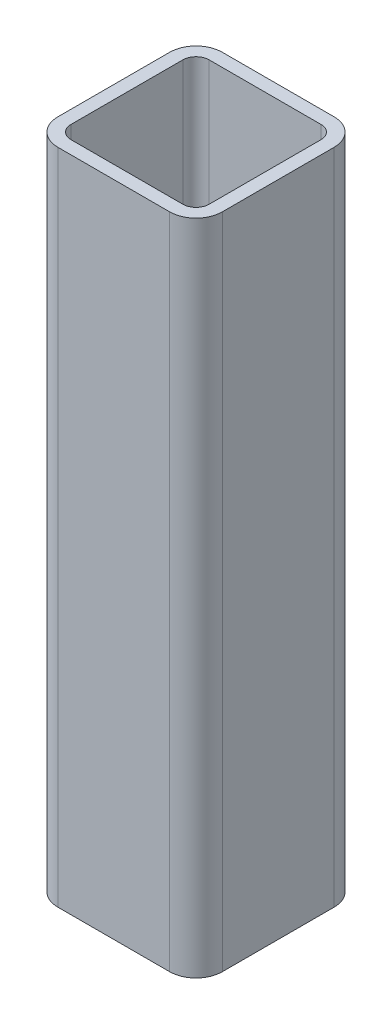
SolidWorks part; units mm, degrees
material "Q235B"
ref_plane "Front Plane" through (0, 0, 0) normal (0, 0, 1) x (1, 0, 0)
ref_plane "Top Plane" through (0, 0, 0) normal (0, 1, 0) x (1, 0, 0)
ref_plane "Right Plane" through (0, 0, 0) normal (1, 0, 0) x (0, 0, -1)
sketch "Sketch1" plane through (0, 0, 0) normal (0, 0, 1) x (1, 0, 0)
  line L0 (0, 0) -> (0, 100)
  dimension "D1" = 100
other "Gb／t 6728—2002 Square hollow section steel 25×2-example.com(1)"
ref_plane "Plane1" through (0, 0, 0) normal (0, 1, 0) x (-1, 0, 0)
sketch "Sketch14" plane through (0, 0, 0) normal (0, 1, 0) x (-1, 0, 0)
  line L0 (-8.5, -10.5) -> (8.5, -10.5)
  line L1 (-10.5, -8.5) -> (-10.5, 8.5)
  line L2 (8.5, 10.5) -> (-8.5, 10.5)
  line L3 (10.5, 8.5) -> (10.5, -8.5)
  line L4 (-8.5, -12.5) -> (8.5, -12.5)
  line L5 (-12.5, -8.5) -> (-12.5, 8.5)
  line L6 (8.5, 12.5) -> (-8.5, 12.5)
  line L7 (12.5, 8.5) -> (12.5, -8.5)
  arc A0 (12.5, 8.5) -> (8.5, 12.5) centre (8.5, 8.5) ccw
  arc A1 (8.5, -12.5) -> (12.5, -8.5) centre (8.5, -8.5) ccw
  arc A2 (-12.5, -8.5) -> (-8.5, -12.5) centre (-8.5, -8.5) ccw
  arc A3 (-8.5, 12.5) -> (-12.5, 8.5) centre (-8.5, 8.5) ccw
  arc A4 (-8.5, 10.5) -> (-10.5, 8.5) centre (-8.5, 8.5) ccw
  arc A5 (10.5, 8.5) -> (8.5, 10.5) centre (8.5, 8.5) ccw
  arc A6 (8.5, -10.5) -> (10.5, -8.5) centre (8.5, -8.5) ccw
  arc A7 (-10.5, -8.5) -> (-8.5, -10.5) centre (-8.5, -8.5) ccw
  point P0 (-12.5, 0)
  point P1 (12.5, 0)
  point P2 (0, 12.5)
  point P3 (0, -12.5)
  point P4 (0, 0)
  point P5 (-12.5, -12.5)
  point P6 (12.5, -12.5)
  point P7 (12.5, 12.5)
  point P8 (-12.5, 12.5)
  point P33 (0, 0)
  dimension "D1" = 4
  dimension "Thickness" = 2
  dimension "V_leg" = 25
